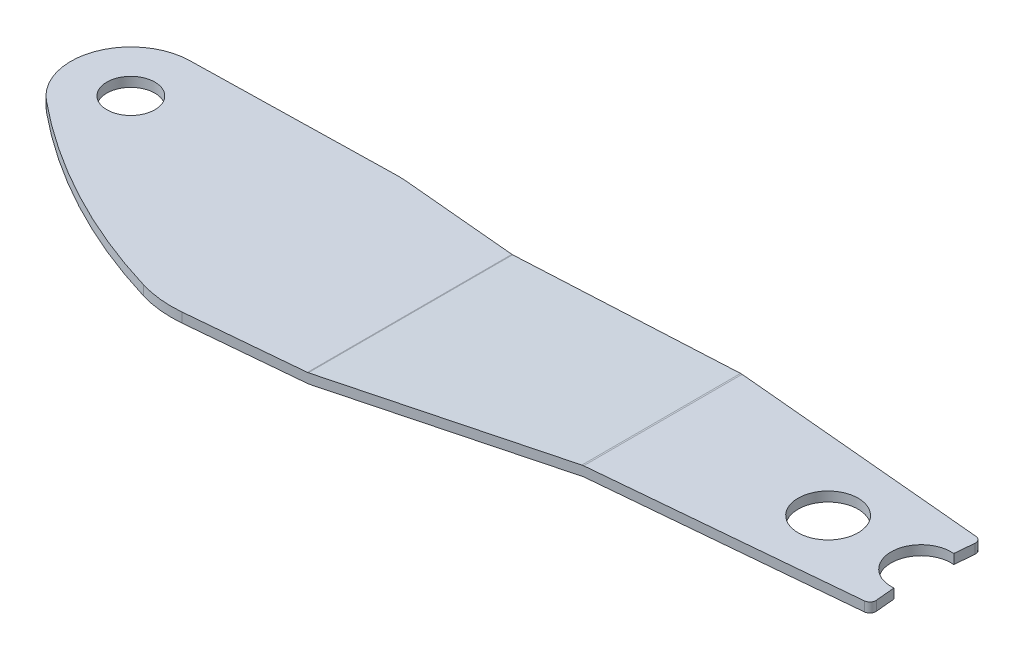
SolidWorks part; units mm, degrees
ref_plane "Front Plane" through (0, 0, 0) normal (0, 0, 1) x (1, 0, 0)
ref_plane "Top Plane" through (0, 0, 0) normal (0, 1, 0) x (1, 0, 0)
ref_plane "Right Plane" through (0, 0, 0) normal (1, 0, 0) x (0, 0, -1)
sketch "Sketch1" plane through (0, 0, 0) normal (0, 0, 1) x (1, 0, 0)
  line L0 (0, 0) -> (-547.3, 0) construction
  line L1 (419.8, 57) -> (851, 57) construction
  line L2 (0, 0) -> (419.8, 57) construction
  line L3 (-1.2164, 8) -> (-647.3, 8)
  line L4 (0.129, 8.0909) -> (417.9201, 64.8182)
  line L5 (420.611, 65) -> (943.5, 65)
  line L6 (-647.3, 8) -> (-647.3, -8)
  line L7 (0, 8) -> (-547.3, 8) construction
  line L8 (943.5, 65) -> (943.5, 49)
  line L9 (419.8, 65) -> (851, 65) construction
  line L10 (421.0164, 49) -> (943.5, 49)
  line L11 (1.8799, -7.8182) -> (419.671, 48.9091)
  line L12 (-0.811, -8) -> (-647.3, -8)
  line L13 (0, -8) -> (-647.3, -8) construction
  line L14 (1.0764, -7.9273) -> (420.8764, 49.0727) construction
  line L15 (-1.0764, 7.9273) -> (418.7236, 64.9273) construction
  line L16 (419.8, 65) -> (943.5, 65) construction
  line L17 (0, 8) -> (-647.3, 8) construction
  line L18 (419.8, 49) -> (943.5, 49) construction
  arc A0 (421.0164, 49) -> (419.671, 48.9091) centre (421.0164, 39) ccw
  arc A1 (0.129, 8.0909) -> (-1.2164, 8) centre (-1.2164, 18) cw
  arc A2 (1.8799, -7.8182) -> (-0.811, -8) centre (-0.811, 12) cw
  arc A3 (420.611, 65) -> (417.9201, 64.8182) centre (420.611, 45) ccw
  dimension "D13" = 10
  dimension "D14" = 20
  dimension "D1" = 547.3
  dimension "D2" = 57
  dimension "D3" = 1398.3
  dimension "D4" = 431.2
  dimension "D8" = 100
  dimension "D9" = 92.5
  dimension "D5" = 8
  dimension "D6" = 8
  dimension "D7" = 8
  dimension "D10" = 16
  dimension "D11" = 16
  dimension "D12" = 16
extrude "Boss-Extrude1" add sketch "Sketch1" along normal blind 600
sketch "Sketch4" plane through (0, 65, 0) normal (0, 1, 0) x (1, 0, 0)
  line L0 (0, 0) -> (0, -1359.8817) construction
  line L1 (-547.3, -1279.6671) -> (-547.3, 561.2691) construction
  line L2 (-647.3, -600) -> (-647.3, 0) construction
  line L3 (-647.3, -300) -> (1324.1271, -300) construction
  line L4 (-647.3, -600) -> (-647.3, 0) construction
  line L5 (-616.4551, -218.5) -> (-263.7468, -218.5) construction
  line L6 (-209.8, -1329.3592) -> (-209.8, 330.295) construction
  line L7 (849.441, -393.0228) -> (-192.7412, -487.7265)
  line L8 (849.441, -206.9772) -> (-192.7412, -112.2735)
  line L9 (-549.3793, -118.5216) -> (-213.7195, -111.5408)
  line L10 (858.495, -217.8412) -> (855.5538, -250.2078)
  line L11 (851, -1009.9733) -> (851, 231.9619) construction
  line L12 (696, -822.7119) -> (696, 170.4845) construction
  line L13 (858.495, -382.1588) -> (855.5538, -349.7922)
  circle A0 centre (-547.3, -218.5) radius 40
  arc A1 (-549.3793, -118.5216) -> (-610.7425, -295.7985) centre (-547.3, -218.5) ccw
  arc A2 (-264.0347, -480.5294) -> (-192.7412, -487.7265) centre (-209.8, -300) ccw
  arc A3 (859.371, -392.1204) -> (859.371, -207.8796) centre (851, -300) ccw construction
  arc A4 (855.5538, -250.2078) -> (855.5538, -349.7922) centre (851, -300) ccw
  circle A5 centre (696, -300) radius 50
  arc A6 (-610.7425, -295.7985) -> (-264.0347, -480.5294) centre (23.6823, 477.1861) ccw
  arc A7 (-192.7412, -112.2735) -> (-213.7195, -111.5408) centre (-209.8, -300) ccw
  arc A8 (858.495, -382.1588) -> (849.441, -393.0228) centre (848.5361, -383.0638) cw
  arc A9 (849.441, -206.9772) -> (858.495, -217.8412) centre (848.5361, -216.9362) cw
  point P40 (859.4, -392.1178)
  point P43 (859.4, -207.8822)
  dimension "D3" = 80
  dimension "D4" = 200
  dimension "D7" = 2000
  dimension "D10" = 185
  dimension "D11" = 100
  dimension "D12" = 100
  dimension "D6" = 377
  dimension "D8" = 8.4
  dimension "D14" = 10
  dimension "D1" = 100
  dimension "D2" = 81.5
  dimension "D5" = 337.5
  dimension "D9" = 1398.3
  dimension "D13" = 155
extrude "Cut-Extrude1" cut sketch "Sketch4" against normal through all flip side to cut
